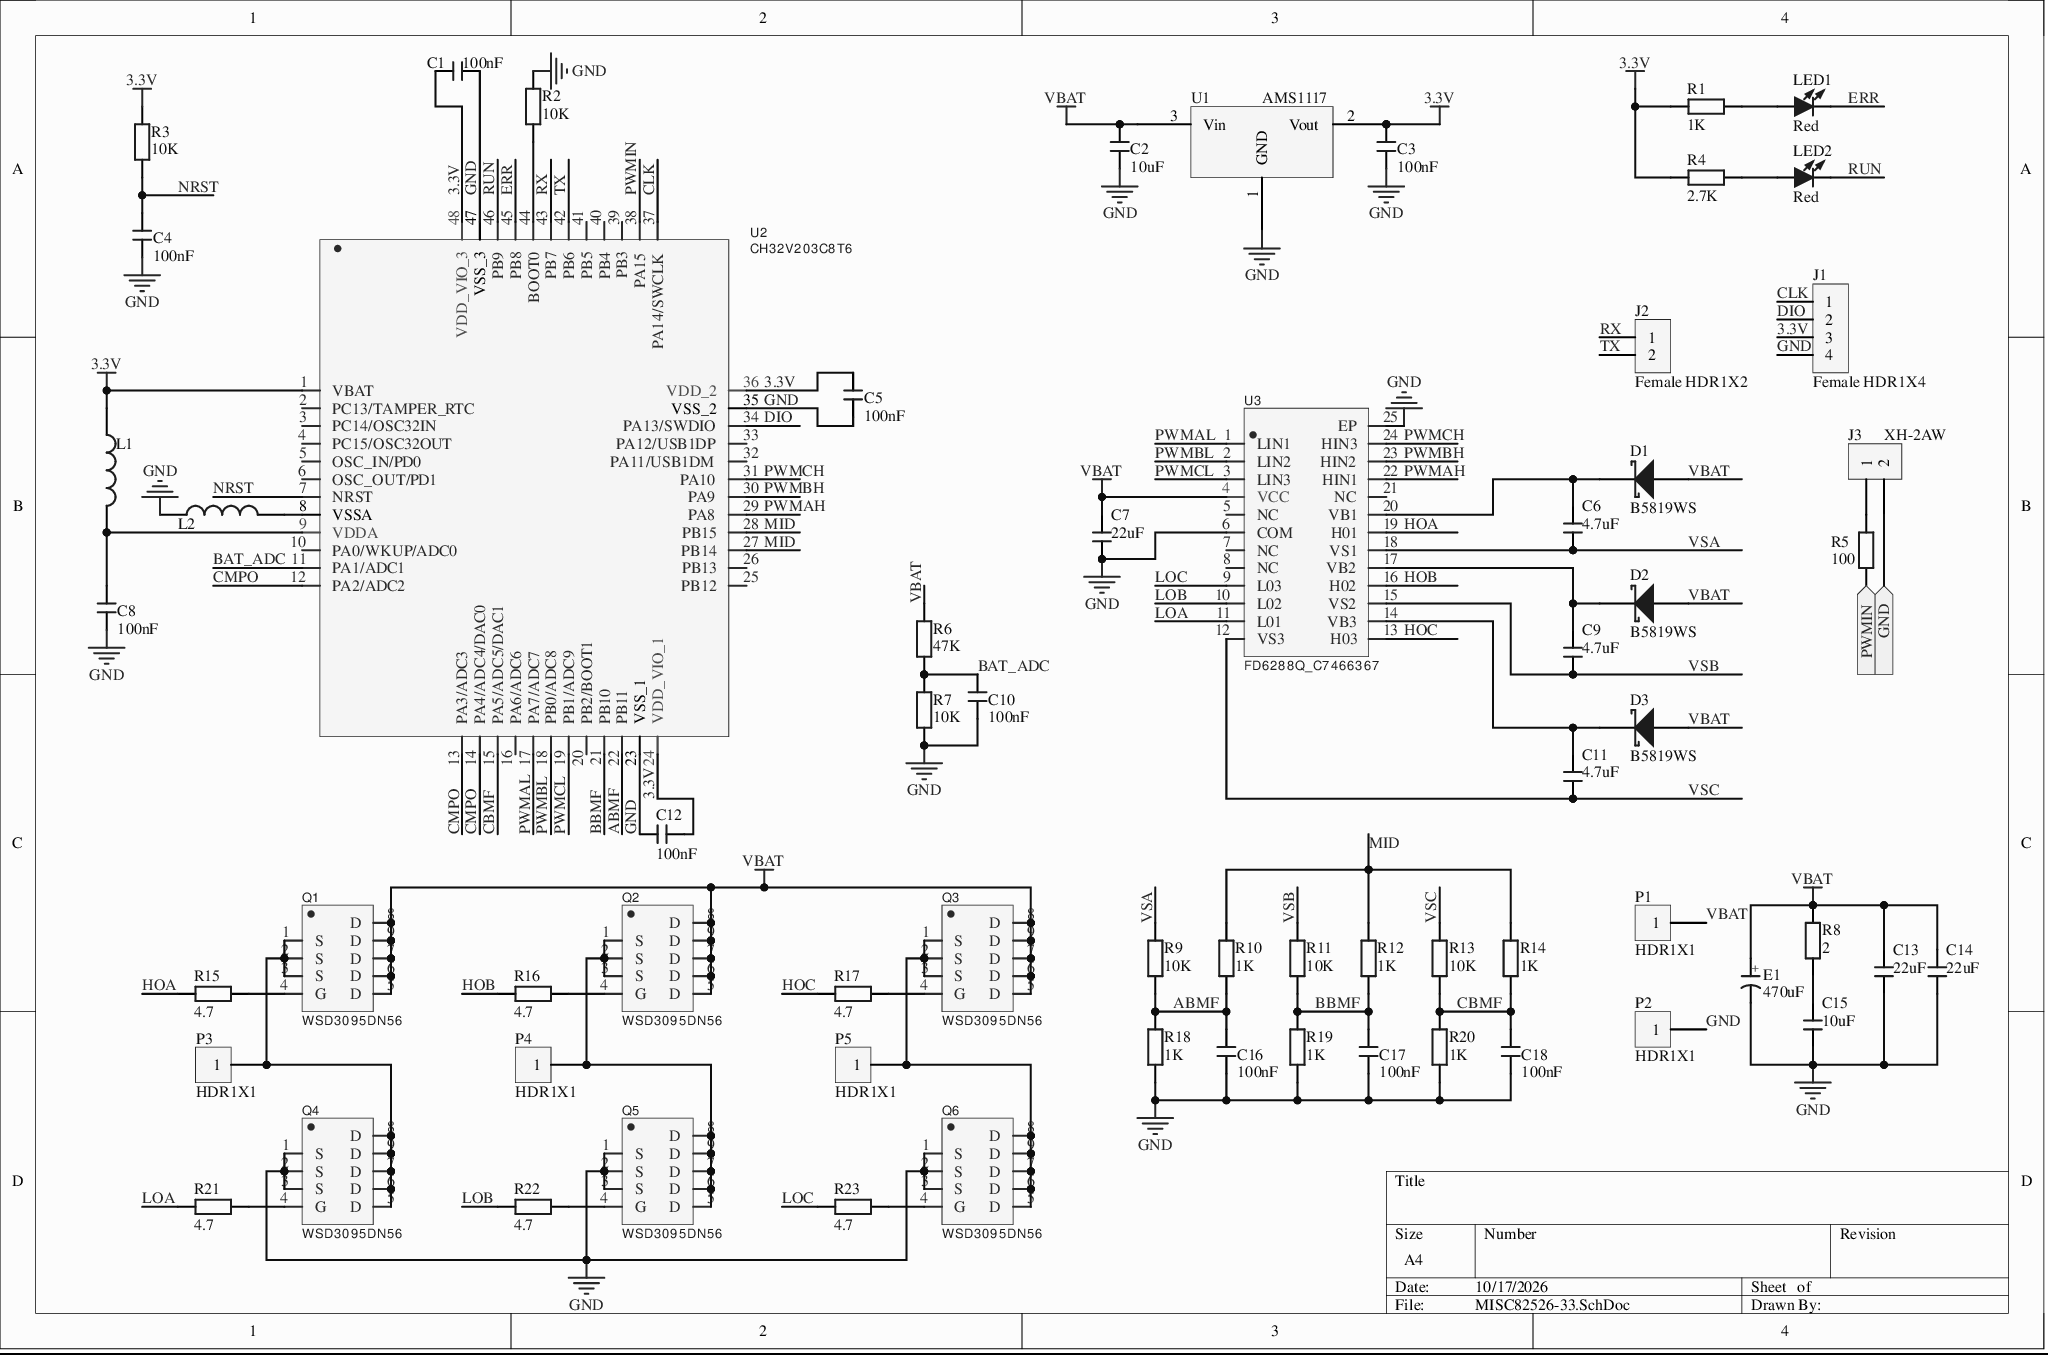
[diagram p0: MISC82526-33.SchDoc]
# Altium project MISC82526-3.PrjPcb
1 sheet, 66 parts. Net scope: flat (ports and power ports of the same name join across sheets).
Board file: MISC82526.PcbDoc

## Sheet MISC82526-33.SchDoc
size A4

### Parts
C1  100nF  [C 0603_L]
C2  10uF  [C 0603_L]
C3  100nF  [C 0603_L]
C4  100nF  [C 0603_L]
C5  100nF  [C 0603_L]
C6  4.7uF  [C 0805_L]
C7  22uF  [C 0805_L]
C8  100nF  [C 0603_L]
C9  4.7uF  [C 0805_L]
C10  100nF  [C 0603_L]
C11  4.7uF  [C 0805_L]
C12  100nF  [C 0603_L]
C13  22uF  [C 0805_L]
C14  22uF  [C 0805_L]
C15  10uF  [C 0805_L]
C16  100nF  [C 0603_L]
C17  100nF  [C 0603_L]
C18  100nF  [C 0603_L]
D1  B5819WS  [SOD-323]
D2  B5819WS  [SOD-323]
D3  B5819WS  [SOD-323]
E1  470uF  [CM A(3*5.4)]
J1  Female HDR1X4  [Fe-HDR1X4/2.54-S]
J2  Female HDR1X2  [Fe-HDR1X2/2.54-S]
J3  XH-2AW  [Fe-HDR1X2/2.54-S]
L1  10uH  [L 0805]  (value not drawn)
L2  10uH  [L 0805]  (value not drawn)
LED1  Red  [LED 0805G]
LED2  Red  [LED 0805G]
P1  HDR1X1  [HDR1X1]
P2  HDR1X1  [HDR1X1]
P3  HDR1X1  [HDR1X1]
P4  HDR1X1  [HDR1X1]
P5  HDR1X1  [HDR1X1]
Q1  WSD3095DN56  [PDFN-8_L5.2-W5.9-P1.27-LS6.2-BL]
Q2  WSD3095DN56  [PDFN-8_L5.2-W5.9-P1.27-LS6.2-BL]
Q3  WSD3095DN56  [PDFN-8_L5.2-W5.9-P1.27-LS6.2-BL]
Q4  WSD3095DN56  [PDFN-8_L5.2-W5.9-P1.27-LS6.2-BL]
Q5  WSD3095DN56  [PDFN-8_L5.2-W5.9-P1.27-LS6.2-BL]
Q6  WSD3095DN56  [PDFN-8_L5.2-W5.9-P1.27-LS6.2-BL]
R1  1K  [R 0603_L]
R2  10K  [R 0603_L]
R3  10K  [R 0603_L]
R4  2.7K  [R 0603_L]
R5  100  [R 0603_L]
R6  47K  [R 0603_L]
R7  10K  [R 0603_L]
R8  2  [R 0603_L]
R9  10K  [R 0603_L]
R10  1K  [R 0603_L]
R11  10K  [R 0603_L]
R12  1K  [R 0603_L]
R13  10K  [R 0603_L]
R14  1K  [R 0603_L]
R15  4.7  [R 0603_L]
R16  4.7  [R 0603_L]
R17  4.7  [R 0603_L]
R18  1K  [R 0603_L]
R19  1K  [R 0603_L]
R20  1K  [R 0603_L]
R21  4.7  [R 0603_L]
R22  4.7  [R 0603_L]
R23  4.7  [R 0603_L]
U1  AMS1117  [SOT223]
U2  CH32V203C8T6  [LQFP-48_L7.0-W7.0-P0.50-LS9.0-BL]
U3  FD6288Q_C7466367  [QFN-24_L4.0-W4.0-P0.50-BL-EP2.7]

### Ports
GND (in), PWMIN (in)

### Nets
3.3V: C1.1 C3.2 C5.2 C12.1 J1.3 L1.1 R1.2 R3.2 R4.2 U1.2(Vout) U2.1(VBAT) U2.24(VDD_VIO_1) U2.36(VDD_2) U2.48(VDD_VIO_3)
GND: C1.2 C2.1 C3.1 C4.1 C5.1 C7.1 C8.1 C10.1 C12.2 C13.1 C14.1 C15.1 C16.1 C17.1 C18.1 E1.2(K) J1.4 L2.1 P2.1 Q4.1(S) Q4.2(S) Q4.3(S) Q5.1(S) Q5.2(S) Q5.3(S) Q6.1(S) Q6.2(S) Q6.3(S) R2.2 R7.1 R18.1 R19.1 R20.1 U1.1(GND) U2.23(VSS_1) U2.35(VSS_2) U2.47(VSS_3) U3.6(COM) U3.25(EP)
VBAT: C2.2 C7.2 C13.2 C14.2 D1.1(A) D2.1(A) D3.1(A) E1.1(A) P1.1 Q1.5(D) Q1.6(D) Q1.7(D) Q1.8(D) Q1.9(D) Q2.5(D) Q2.6(D) Q2.7(D) Q2.8(D) Q2.9(D) Q3.5(D) Q3.6(D) Q3.7(D) Q3.8(D) Q3.9(D) R6.2 R8.2 U1.3(Vin) U3.4(VCC)
ABMF: C16.2 R9.1 R10.1 R18.2 U2.22(PB11)
BAT_ADC: C10.2 R6.1 R7.2 U2.11(PA1/ADC1)
BBMF: C17.2 R11.1 R12.1 R19.2 U2.21(PB10)
CBMF: C18.2 R13.1 R14.1 R20.2 U2.15(PA5/ADC5/DAC1)
CLK: J1.1 U2.37(PA14/SWCLK)
CMPO: U2.12(PA2/ADC2) U2.13(PA3/ADC3) U2.14(PA4/ADC4/DAC0)
DIO: J1.2 U2.34(PA13/SWDIO)
ERR: LED1.2(K) U2.45(PB8)
HOA: R15.2 U3.19(H01)
HOB: R16.2 U3.16(H02)
HOC: R17.2 U3.13(H03)
LOA: R21.2 U3.11(L01)
LOB: R22.2 U3.10(L02)
LOC: R23.2 U3.9(L03)
MID: R10.2 R12.2 R14.2 U2.27(PB14) U2.28(PB15)
NRST: C4.2 R3.1 U2.7(NRST)
PWMAH: U2.29(PA8) U3.22(HIN1)
PWMAL: U2.17(PA7/ADC7) U3.1(LIN1)
PWMBH: U2.30(PA9) U3.23(HIN2)
PWMBL: U2.18(PB0/ADC8) U3.2(LIN2)
PWMCH: U2.31(PA10) U3.24(HIN3)
PWMCL: U2.19(PB1/ADC9) U3.3(LIN3)
PWMIN: U2.38(PA15)
RUN: LED2.2(K) U2.46(PB9)
RX: J2.1 U2.43(PB7)
TX: J2.2 U2.42(PB6)
VSA: C6.1 R9.2 U3.18(VS1)
VSB: C9.1 R11.2 U3.15(VS2)
VSC: C11.1 R13.2 U3.12(VS3)
NetC6_2: C6.2 D1.2(K) U3.20(VB1)
NetC8_2: C8.2 L1.2 U2.9(VDDA)
NetC9_2: C9.2 D2.2(K) U3.17(VB2)
NetC11_2: C11.2 D3.2(K) U3.14(VB3)
NetC15_2: C15.2 R8.1
NetJ3_1: J3.1 R5.1
NetJ3_2: J3.2 ; port GND
NetL2_2: L2.2 U2.8(VSSA)
NetLED1_1: LED1.1(A) R1.1
NetLED2_1: LED2.1(A) R4.1
NetP3_1: P3.1 Q1.1(S) Q1.2(S) Q1.3(S) Q4.5(D) Q4.6(D) Q4.7(D) Q4.8(D) Q4.9(D)
NetP4_1: P4.1 Q2.1(S) Q2.2(S) Q2.3(S) Q5.5(D) Q5.6(D) Q5.7(D) Q5.8(D) Q5.9(D)
NetP5_1: P5.1 Q3.1(S) Q3.2(S) Q3.3(S) Q6.5(D) Q6.6(D) Q6.7(D) Q6.8(D) Q6.9(D)
NetQ1_4: Q1.4(G) R15.1
NetQ2_4: Q2.4(G) R16.1
NetQ3_4: Q3.4(G) R17.1
NetQ4_4: Q4.4(G) R21.1
NetQ5_4: Q5.4(G) R22.1
NetQ6_4: Q6.4(G) R23.1
NetR2_1: R2.1 U2.44(BOOT0)
NetR5_2: R5.2 ; port PWMIN

Not connected (* = marked no-connect by the designer): U2 2(PC13/TAMPER_RTC)* 3(PC14/OSC32IN)* 4(PC15/OSC32OUT)* 5(OSC_IN/PD0)* 6(OSC_OUT/PD1)* 10(PA0/WKUP/ADC0)* 16(PA6/ADC6)* 20(PB2/BOOT1)* 25(PB12)* 26(PB13)* 32(PA11/USB1DM)* 33(PA12/USB1DP)* 39(PB3)* 40(PB4)* 41(PB5)*; U3 5(NC)* 7(NC)* 8(NC)* 21(NC)*

### Library data of the parts
C1-C18 = C: SMD capacitor; BOM名称: Non-polar SMD capacitor; xxxxxxxxxxxxxxxxxxxxxxxxxxx: -
D1-D3 = 1N5819: Schottky diode; 属性: 40V/2A; BOM名称: Schottky diode; xxxxxxxxxxxxxxxxxxxxxxxxxxx: -
E1 = CE_SMD: SMD electrolytic capacitor; BOM名称: SMD electrolytic capacitor; xxxxxxxxxxxxxxxxxxxxxxxxxxx: -
J3 = Female HDR1X2
L1 L2 = L: Low-power SMD inductor; BOM名称: Low-power SMD inductor; xxxxxxxxxxxxxxxxxxxxxxxxxxx: -
LED1 LED2 = LED-SMD: SMD LED; BOM名称: SMD LED; xxxxxxxxxxxxxxxxxxxxxxxxxxx: -
R1-R23 = R: SMD resistor; BOM名称: SMD resistor; xxxxxxxxxxxxxxxxxxxxxxxxxxx: -
U1 = AMS1117: Three-terminal voltage regulator